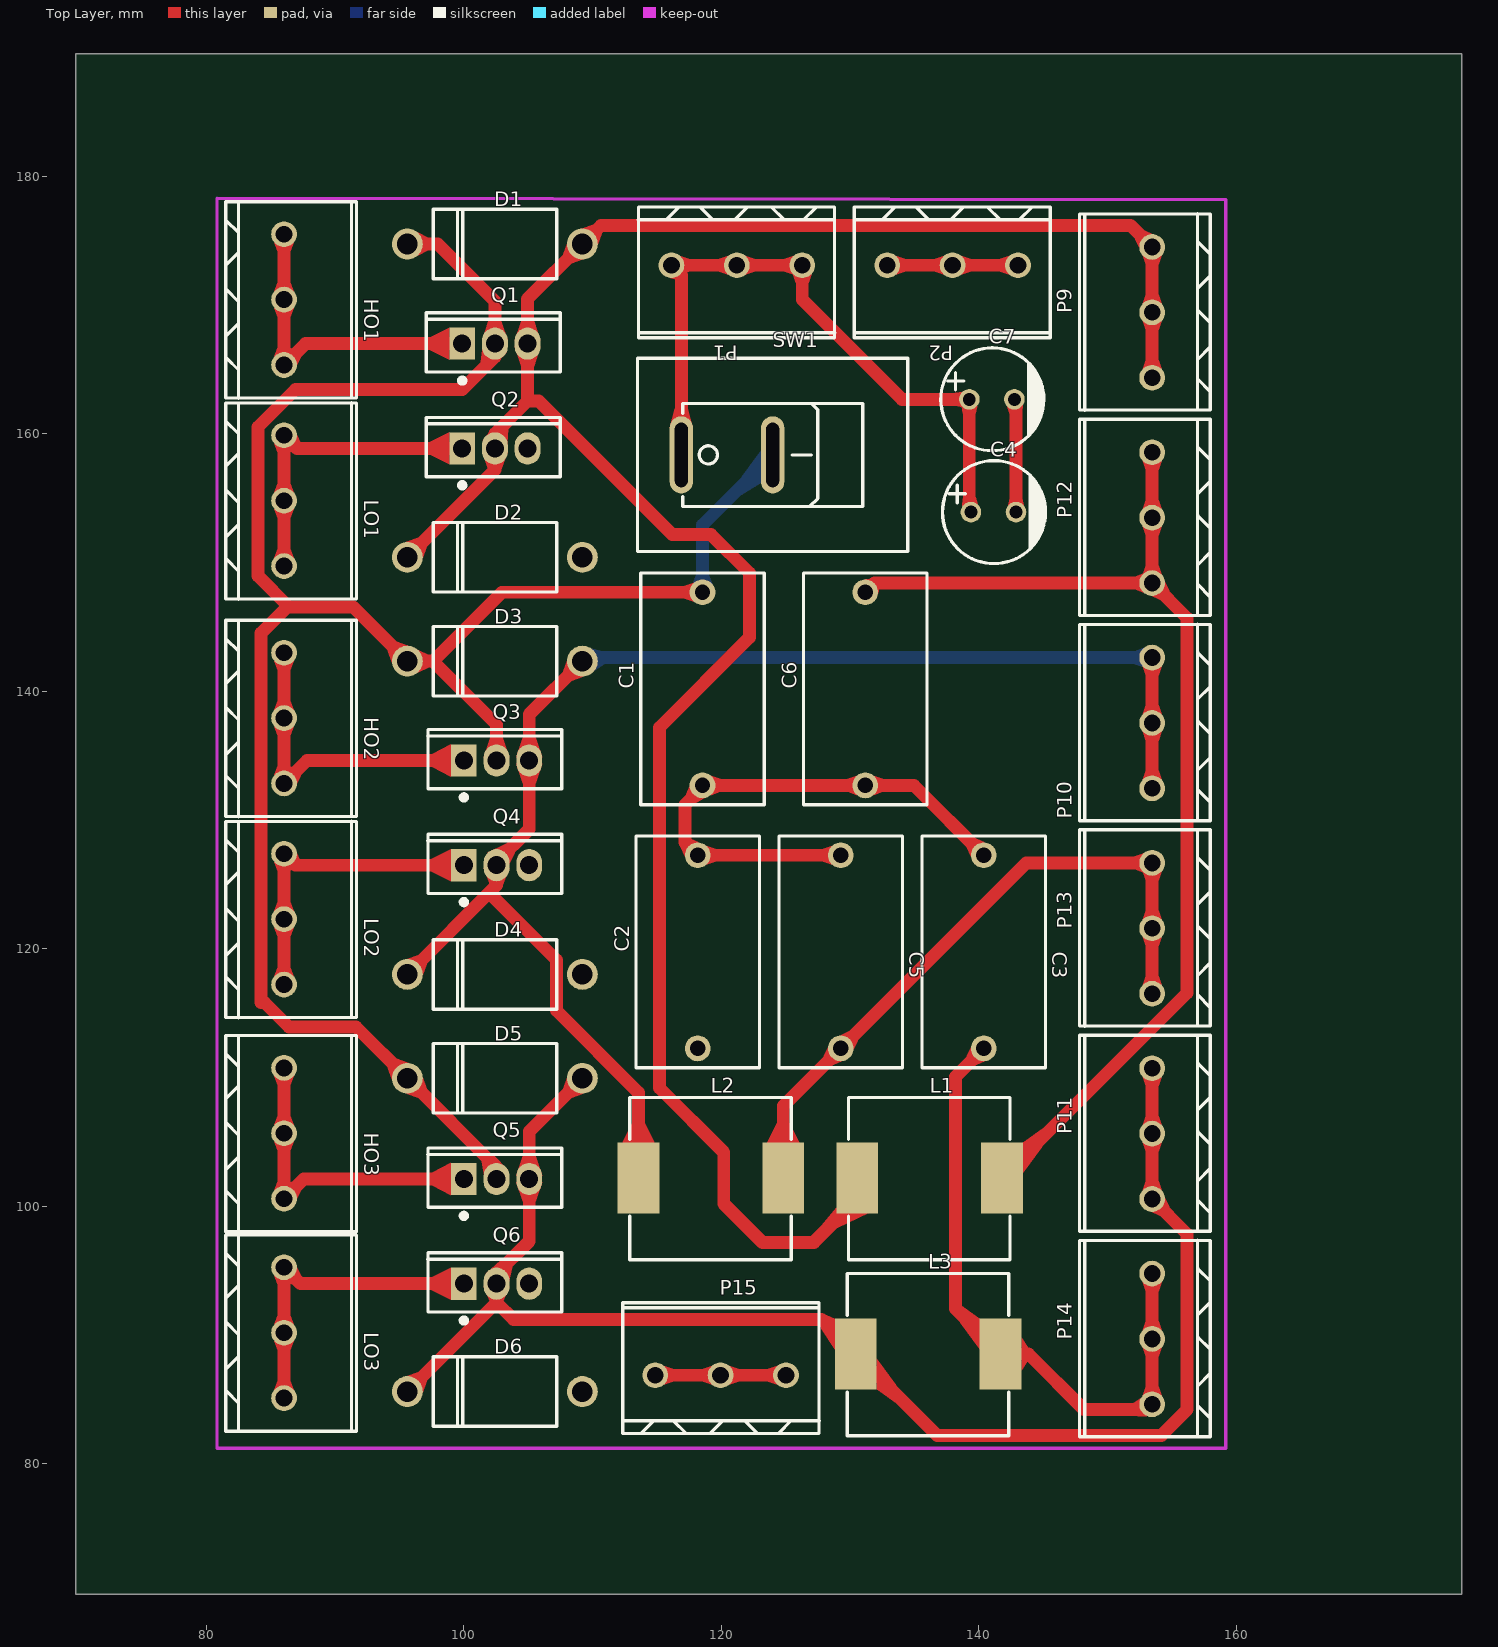
[diagram p0: Top Layer view]
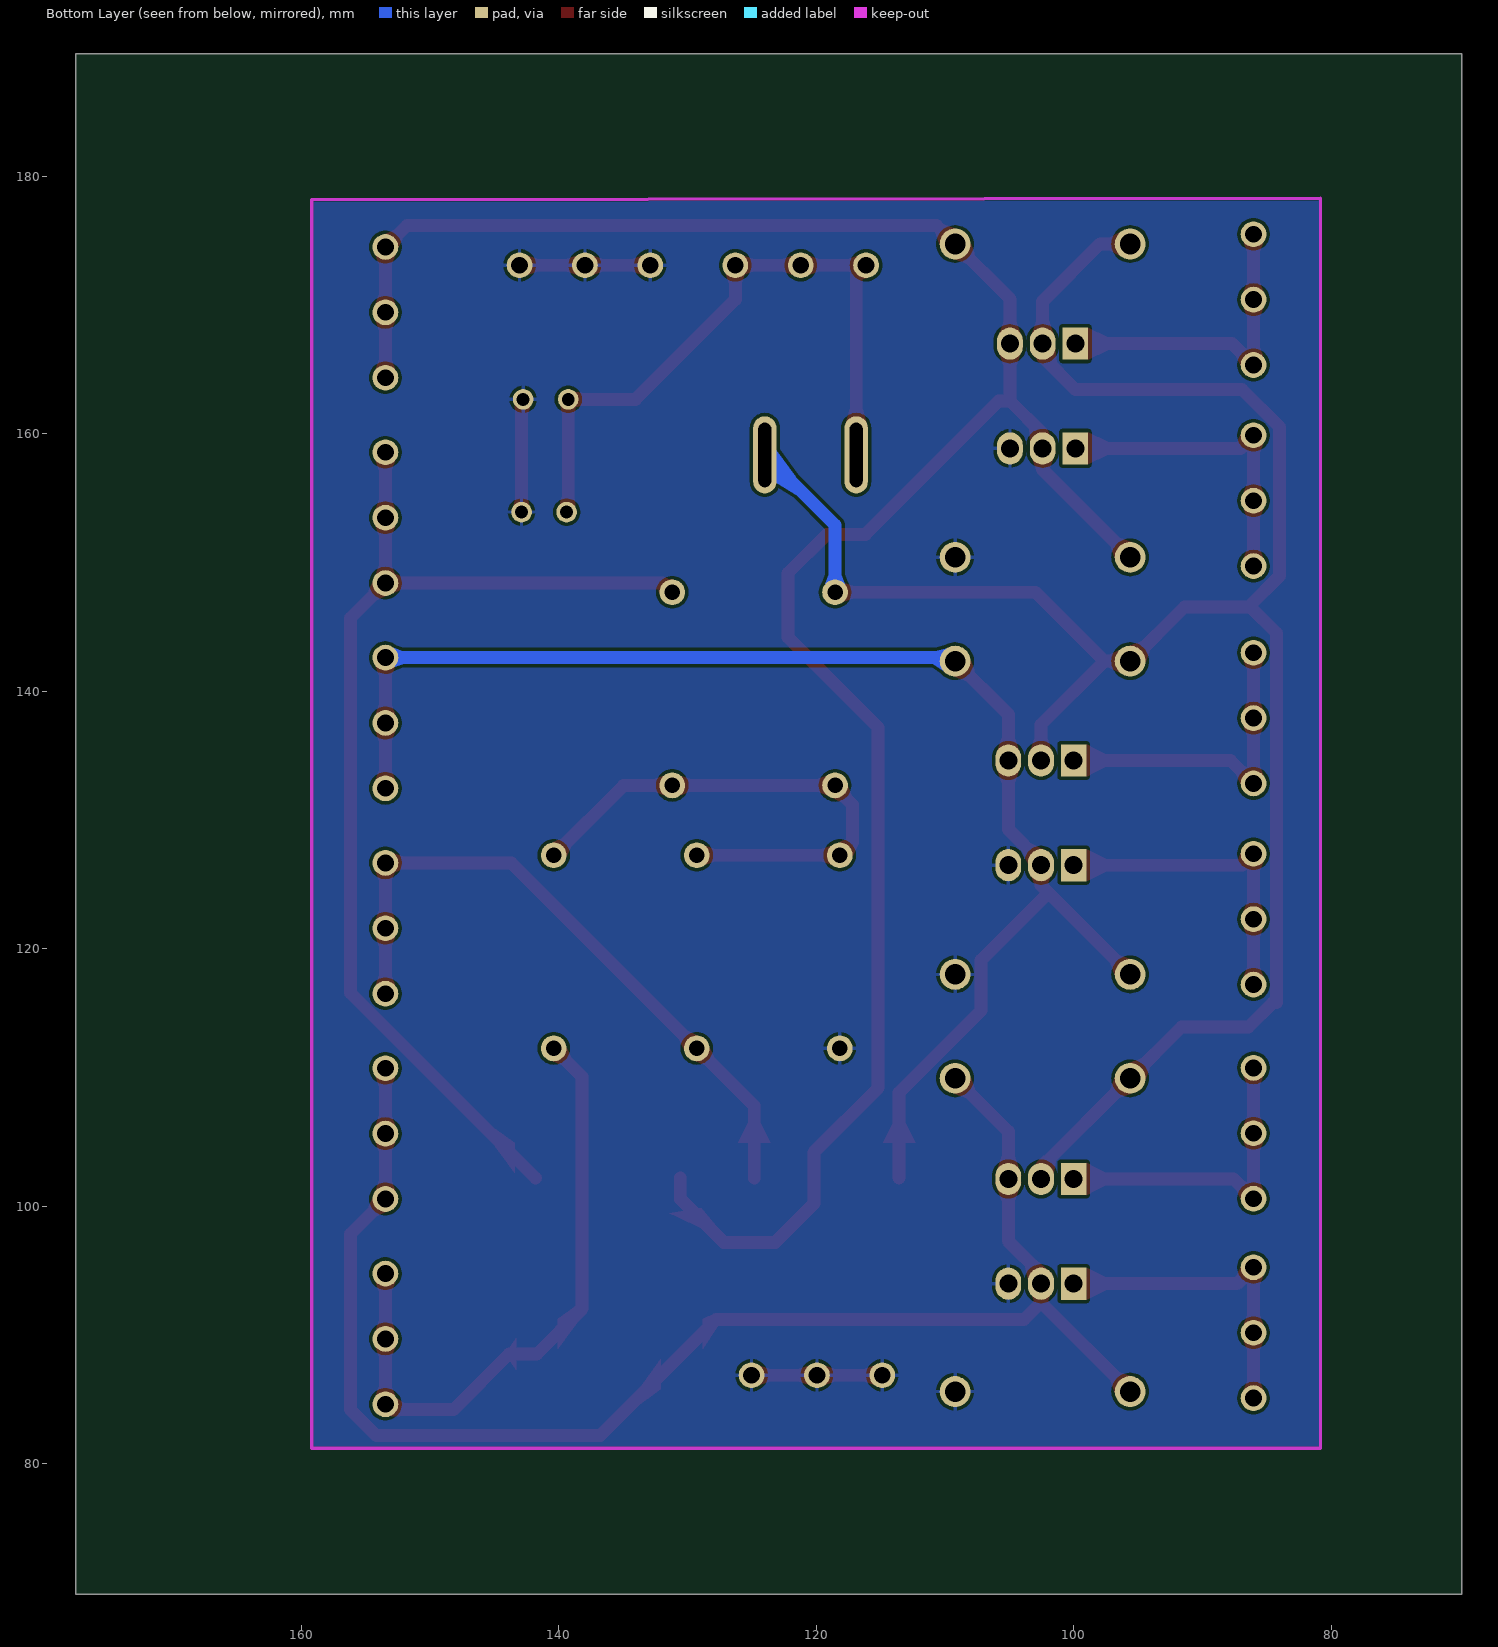
[diagram p1: Bottom Layer view, seen from below]
# Altium PCB MISC75150.pcbdoc
Units mm, origin at the board's own origin, x right, y up, seen from the top; angles counter-clockwise.
Board outline 107.7 x 119.7 mm, 2 copper layers (Top Layer, Bottom Layer), stack 0.07 mm thick; 38 components, 16 nets, 97 pads, 0 vias.

## Layer stack, top to bottom
Top Solder Mask Layer: solder mask 0.01, Dk 3.3
Top Layer: signal copper 0.035
Bottom Layer: signal copper 0.035
Bottom Solder Mask Layer: solder mask 0.01, Dk 3.3

## Board outline
177.55,69.85 69.85,69.85 69.85,189.55 177.55,189.55

## Design rules (kind name [scope] priority, off if disabled: settings)
BoardOutlineClearance Default_1 [All] p2: genericclearance=0.102 ignorepadtopadclearanceinfootprint=FALSE except(0: Arc-SplitContinuation Track-SplitContinuation SMDPad-SplitContinuation THPad-SplitContinuation Via-SplitContinuation Fill-SplitContinuation Region-SplitContinuation Poly-SplitContinuation Text-SplitContinuation Hole-SplitContinuation; 0.152: Arc-OutlineEdge Track-OutlineEdge SMDPad-OutlineEdge THPad-OutlineEdge Via-OutlineEdge Fill-OutlineEdge Region-OutlineEdge Poly-OutlineEdge Text-OutlineEdge Hole-OutlineEdge SMDPad-CutoutEdge THPad-CutoutEdge Via-CutoutEdge Fill-CutoutEdge Region-CutoutEdge Text-CutoutEdge; 0.175: Hole-CutoutEdge; 0.254: Poly-CutoutEdge; 0.3: Arc-CutoutEdge Track-CutoutEdge)
Clearance Default [All] p1: gap=0.102 ignorepadtopadclearanceinfootprint=FALSE except(0.152: SMDPad-Track SMDPad-SMDPad THPad-Track SMDPad-THPad THPad-THPad Track-Via SMDPad-Via THPad-Via Via-Via Fill-Track Region-Track Fill-SMDPad Region-SMDPad Fill-THPad Region-THPad Fill-Via Region-Via Fill-Fill Fill-Region Region-Region Arc-Track Arc-SMDPad Arc-THPad Arc-Via Fill-Arc Region-Arc Arc-Arc Text-Track SMDPad-Text Text-THPad Text-Via Fill-Text Region-Text Arc-Text Text-Text; 0.175: Hole-Track Hole-SMDPad Hole-THPad Hole-Via Fill-Hole Region-Hole Hole-Arc Hole-Text; 0.254: Poly-Track Poly-SMDPad Poly-THPad Poly-Via Poly-Fill Poly-Region Poly-Poly Poly-Arc Poly-Text Poly-Hole)
DiffPairsRouting differentialPair [All] p1: maxlimit=0.152 minlimit=0.127 mostfreqgap=0.152 toplayer_minwidth=0.127 toplayer_prefwidth=2.54 toplayer_maxwidth=2.54 toplayer_mingap=0.127 toplayer_prefgap=0.152 toplayer_maxgap=0.152 bottomlayer_minwidth=0.127 bottomlayer_prefwidth=2.54 bottomlayer_maxwidth=2.54 bottomlayer_mingap=0.127 bottomlayer_prefgap=0.152 bottomlayer_maxgap=0.152 maxuncoupledlength=0.254
HoleToHoleClearance otherClearance [All] p1: gap=0.3 allowstackedmicrovias=TRUE
Length netLength [All] p1: minlimit=0 maxlimit=0
MatchedLengths netLengthTolerance [All] p1: tolerance=25.4
PasteMaskExpansion pasteMaskExpansion [All] p1: expansion=0
PlaneConnect innerPlane [All] p1: planeconnectstyle=Relief reliefexpansion=0.508 reliefentries=4 reliefconductorwidth=0.254 reliefairgap=0.254
PolygonConnect copperRegion [All] p1: connectstyle=Relief reliefconductorwidth=0.254 reliefentries=4 polygonreliefangle="90 Angle" airgapwidth=0.254 via.connectstyle=Relief via.reliefconductorwidth=0.254 via.reliefentries=4 via.polygonreliefangle="90 Angle" via.airgapwidth=0.254
RoutingVias Default_3 [All] p1: holewidth=0.305 width=0.61 viastyle="Through Hole" minholewidth=0.305 minwidth=0.61 maxholewidth=29.997 maxwidth=50.013
SolderMaskExpansion Common [IsVia] p1: expansion=-25.4 istentingtop=TRUE
SolderMaskExpansion Common [All] p2: expansion=0.051 istentingtop=FALSE
Width Default_2 [All] p1: maxlimit=25.4 minlimit=0.254 preferedwidth=0.254

## Components (designator, comment, footprint, x,y, rotation, side; value= is the part's Value field where it differs from the comment)
C1 "1uF" CAP-TH_L18.0-W9.5-P15.00-D1.2 118.551,140.2 r90 top
C2 "1uF" CAP-TH_L18.0-W9.5-P15.00-D1.2 118.18,119.768 r90 top
C3 "1uF" CAP-TH_L18.0-W9.5-P15.00-D1.2 140.405,119.768 r270 top
C4 "100uF, voltage stabilising" CAP-TH_BD8.0-P3.50-D1.0-FD 141.157,153.931 r0 top
C5 "1uF" CAP-TH_L18.0-W9.5-P15.00-D1.2 129.293,119.768 r270 top
C6 "1uF" CAP-TH_L18.0-W9.5-P15.00-D1.2 131.2,140.2 r90 top
C7 "100uF, voltage stabilising" CAP-TH_BD8.0-P3.50-D1.0-FD 141.03,162.694 r0 top
D1 "FR307" DO-201AD_BD5.3-L8.4-P12.50-D1.4-RD 102.422,174.759 r0 top
D2 "FR307" DO-201AD_BD5.3-L8.4-P12.50-D1.4-RD 102.422,150.42 r0 top
D3 "FR307" DO-201AD_BD5.3-L8.4-P12.50-D1.4-RD 102.422,142.352 r0 top
D4 "FR307" DO-201AD_BD5.3-L8.4-P12.50-D1.4-RD 102.422,118.012 r0 top
D5 "FR307" DO-201AD_BD5.3-L8.4-P12.50-D1.4-RD 102.422,109.944 r0 top
D6 "FR307" DO-201AD_BD5.3-L8.4-P12.50-D1.4-RD 102.422,85.605 r0 top
HO1 "First channel high-level control input" CONN-TH_3P-P5.00_WJ500V-5.08-3P 86.039,170.441 r270 top
HO2 "Second channel high-level control input" CONN-TH_3P-P5.00_WJ500V-5.08-3P 86.039,137.929 r270 top
HO3 "Third channel high-level control input" CONN-TH_3P-P5.00_WJ500V-5.08-3P 86.039,105.671 r270 top
L1 "100uH" IND-SMD_L13.5-W12.6_125CDMCC-DS 136.2,102.2 r0 top
L2 "100uH" IND-SMD_L13.5-W12.6_125CDMCC-DS 119.2,102.2 r0 top
L3 "100uH" IND-SMD_L13.5-W12.6_125CDMCC-DS 136.087,88.526 r0 top
LO1 "First channel low-level control input" CONN-TH_3P-P5.00_WJ500V-5.08-3P 86.039,154.82 r270 top
LO2 "Second channel low-level control input" CONN-TH_3P-P5.00_WJ500V-5.08-3P 86.039,122.308 r270 top
LO3 "Third channel low-level control input" CONN-TH_3P-P5.00_WJ500V-5.08-3P 86.039,90.177 r270 top
P1 "DC supply V1 positive" CONN-TH_3P-P5.00_WJ500V-5.08-3P 121.218,173.108 r180 top
P2 "DC supply V1 negative" CONN-TH_3P-P5.00_WJ500V-5.08-3P 137.982,173.108 r180 top
P9 "Provides first channel reference voltage" CONN-TH_3P-P5.00_WJ500V-5.08-3P 153.486,169.45 r90 top
P10 "Provides second channel reference voltage" CONN-TH_3P-P5.00_WJ500V-5.08-3P 153.486,137.548 r90 top
P11 "Provides third channel reference voltage" CONN-TH_3P-P5.00_WJ500V-5.08-3P 153.486,105.646 r90 top
P12 "First channel load" CONN-TH_3P-P5.00_WJ500V-5.08-3P 153.486,153.499 r90 top
P13 "Second channel load" CONN-TH_3P-P5.00_WJ500V-5.08-3P 153.486,121.597 r90 top
P14 "Third channel load" CONN-TH_3P-P5.00_WJ500V-5.08-3P 153.486,89.694 r90 top
P15 "Add ground interface" CONN-TH_3P-P5.00_WJ500V-5.08-3P 119.958,86.875 r0 top
Q1 "IRF540N" TO-220AB-3_L10.4-W4.6-P2.54-L 102.422,167.019 r0 top
Q2 "IRF540N" TO-220AB-3_L10.4-W4.6-P2.54-L 102.422,158.884 r0 top
Q3 "IRF540N" TO-220AB-3_L10.4-W4.6-P2.54-L 102.549,134.634 r0 top
Q4 "IRF540N" TO-220AB-3_L10.4-W4.6-P2.54-L 102.549,126.499 r0 top
Q5 "IRF540N" TO-220AB-3_L10.4-W4.6-P2.54-L 102.549,102.122 r0 top
Q6 "IRF540N" TO-220AB-3_L10.4-W4.6-P2.54-L 102.549,93.987 r0 top
SW1 "MR1-110-C5N-BB" SW-TH_MR1-110-C5N-BB 120.456,158.376 r0 top

## Footprints (in the part's own frame and the unit in brackets; to place one, negate y for a bottom-side part, rotate by r counter-clockwise, add the part's x,y. Pads: shape width x height; smd on the part's side, far side on the other; paste and mask are expansions set on the pad)
CAP-TH_BD8.0-P3.50-D1.0-FD [mm]
  round 1.6 hole 1 paste+0 mask+0.102: 1(-1.75,0) 2(1.75,0)
  Top Layer circle w0.6: c1.75,0 r0.3
  Top Layer circle w0.6: c-1.75,0 r0.3
  silkscreen extent -3.96,-4 4.04,4
CAP-TH_L18.0-W9.5-P15.00-D1.2 [mm]
  round 2 hole 1.2 paste+0 mask+0.102: 1(-7.501,0) 2(7.501,0)
  silkscreen extent -9,-4.8 9,4.8
CONN-TH_3P-P5.00_WJ500V-5.08-3P [mm]
  round 2 hole 1.3 paste+0 mask+0.102: 1(-5.08,0) 2(0,0) 3(5.08,0)
  silkscreen extent -7.61,-4.53 7.66,5.64
DO-201AD_BD5.3-L8.4-P12.50-D1.4-RD [mm]
  round 2.4 hole 1.6 paste+0 mask+0.102: 1(-6.8,0) 2(6.8,0)
  silkscreen extent -4.8,-2.7 4.8,2.7
IND-SMD_L13.5-W12.6_125CDMCC-DS [mm]
  rect 3.25x5.5 smd paste+0 mask+0.102: 1(-5.625,0) 2(5.625,0)
  silkscreen extent -6.3,-6.35 6.25,6.25
SW-TH_MR1-110-C5N-BB [mm]
  oval 1.8x6 hole 1 slot 5 at 90 deg paste+0 mask+0.102: 1(-3.55,0) 2(3.55,0)
  silkscreen extent -6.95,-7.5 14.05,7.5
TO-220AB-3_L10.4-W4.6-P2.54-L [mm]
  rect 2x2.5 hole 1.4 paste+0 mask+0.102: 1(-2.54,0)
  oval 2x2.5 hole 1.4 paste+0 mask+0.102: 2(0,0) 3(2.54,0)
  silkscreen extent -5.33,-3.07 5.08,2.4

## Nets (pads, with @x,y where several pads share a name; then routed paths per layer and width w, separated by ;. In a path a pad name is that pad's centre, name@x,y a point inside that pad or via, vN(x,y) a via of type N, cw(c..) or ccw(c..) an arc to the next point about the centre after c; other vN are vias at no path point)
C1_1: C1.1 C2.2 C3.1 C5.1 C6.1 | length 41.6
  Top Layer w1: C5.1 C2.2 117.2,128.249 117.2,131.2 118.551,132.551 C1.1 C6.1 134.974,132.699 C3.1
C1_2: C1.2 D1.1 D3.1 D5.1 Q1.2 Q3.2 Q5.2 SW1.2 | length 163.6
  Top Layer w1: D5.1 91.64,113.926 86.42,113.926 84.515,115.831 84.261,115.831 84.261,144.533 86.293,146.565 86.42,146.565 ; D5.1 102.549,103.017 Q5.2 ; D1.1 97.977,174.759 102.422,170.314 Q1.2 102.422,165.996 99.882,163.456 86.928,163.456 84.007,160.535 84.007,148.978 86.42,146.565 ; 97.619,142.352 102.968,147.701 C1.2 ; Q3.2 102.549,137.421 97.619,142.351 D3.1 91.409,146.565 86.42,146.565
  Bottom Layer w1: C1.2 118.551,152.92 SW1.2@124.007,158.376
C3_2: C3.2 L3.2 P14.1 P14.2 P14.3 | length 50
  Top Layer w1: C3.2 138.201,110.063 138.201,92.039 L3.2 143.875,88.526 148.201,84.2 153.073,84.2 P14.1 ; P14.1 P14.2 P14.3
C5_2: C5.2 L2.2 P13.1 P13.2 P13.3 | length 52.2
  Top Layer w1: L2.2 124.825,107.8 C5.2 ; C5.2 143.702,126.677 P13.3 P13.2 P13.1
C6_2: C6.2 L1.2 P12.1 P12.2 P12.3 | length 86
  Top Layer w1: C6.2 131.919,148.419 P12.1 P12.2 P12.3 ; L1.2 156.199,116.575 156.199,145.704 P12.1
GND: C2.1 C4.2 C7.2 D2.2 D4.2 D6.2 P2.1 P2.2 P2.3 P15.1 P15.2 P15.3 Q2.3 Q4.3 Q6.3 | length 29.1
  Top Layer w1: P15.1 P15.2 P15.3 ; P2.3 P2.2 P2.1 ; C7.2 142.908,162.567 C4.2
Q1_1: HO1.1 HO1.2 HO1.3 Q1.1 | length 24.7
  Top Layer w1: HO1.1 86.039,172.763 HO1.2 HO1.3 87.698,167.02 Q1.1
Q1_3: D1.2 D2.1 L1.1 P9.1 P9.2 P9.3 Q1.3 Q2.2 | length 177.1
  Top Layer w1: D2.1@95.623,150.421 102.422,157.22 Q2.2 102.422,160.027 104.962,162.567 ; L1.1@130.576,102.199 130.576,100.576 127.2,97.2 123.2,97.2 120.2,100.2 120.2,104.2 115.201,109.199 115.201,137.2 122.199,144.2 122.199,149.199 119.199,152.201 116.199,152.201 105.834,162.567 104.962,162.567 ; P9.1 P9.2 P9.3 151.816,176.2 110.664,176.2 D1.2 104.962,170.499 Q1.3 104.962,162.567
Q2_1: LO1.1 LO1.2 LO1.3 Q2.1 | length 24.4
  Top Layer w1: LO1.3 LO1.2 LO1.1 87.055,158.884 Q2.1
Q3_1: HO2.1 HO2.2 HO2.3 Q3.1 | length 24.9
  Top Layer w1: HO2.1 HO2.3 87.825,134.635 Q3.1
Q3_3: D3.2 D4.1 L2.1 P10.1 P10.2 P10.3 Q3.3 Q4.2 | length 111.5
  Top Layer w1: D4.1 102.549,124.939 Q4.2 102.549,126.753 105.089,129.293 Q3.3 105.089,138.219 D3.2 ; 101.97,124.36 107.2,119.13 107.2,115.201 113.576,108.826 L2.1 ; P10.1 P10.2 P10.3
  Bottom Layer w1: D3.2 109.499,142.628 P10.3
Q4_1: LO2.1 LO2.2 LO2.3 Q4.1 | length 24.5
  Top Layer w1: LO2.3 LO2.2 LO2.1 86.928,126.499 Q4.1
Q5_1: HO3.1 HO3.2 HO3.3 Q5.1 | length 24.8
  Top Layer w1: HO3.1 HO3.2 HO3.3 87.571,102.123 Q5.1
Q5_3: D5.2 D6.1 L3.1 P11.1 P11.2 P11.3 Q5.3 Q6.2 | length 116.4
  Top Layer w1: D6.1 102.549,92.532 ; D5.2 105.089,105.811 Q5.3 105.089,97.289 102.549,94.749 Q6.2 102.549,92.532 ; P11.1 P11.2 P11.3 ; P11.1 156.199,97.853 156.199,84.2 154.2,82.199 136.789,82.199 L3.1 127.787,91.201 103.88,91.201 102.549,92.532
Q6_1: LO3.1 LO3.2 LO3.3 Q6.1 | length 24.7
  Top Layer w1: LO3.3 LO3.2 LO3.1 87.309,93.987 Q6.1
VCC: C4.1 C7.1 P1.1 P1.2 P1.3 SW1.1 | length 52.9
  Top Layer w1: SW1.1 116.906,172.341 P1.3 P1.2 P1.1 126.298,170.441 134.045,162.694 C7.1 139.28,154.058 C4.1

## Polygon pours and split planes (outlines as drawn)
GND on Bottom Layer (solid, remove dead copper, pour order 2): 76.2,183.2 171.2,183.2 170.2,182.2 170.2,76.2 76.2,76.2 76.2,77.2

## Keep-outs
Board Outline Layer:
  lines w0.254: 80.832,81.211 159.2,81.2 159.2,178.2 80.832,178.315 80.832,81.211

## Other copper
Top Layer:
  region net VCC: 116.8,172.358 116.8,173.858 117.5,173.608 117.5,172.608
  region net VCC: 116.076,172.11 117.136,173.171 117.26,172.694 116.553,171.987
  region net VCC: 121.88,172.358 121.88,173.858 122.58,173.608 122.58,172.608
  region net VCC: 120.557,172.358 120.557,173.858 119.857,173.608 119.857,172.608
  region net VCC: 125.637,172.358 125.637,173.858 124.937,173.608 124.937,172.608
  region net VCC: 127.048,172.447 125.548,172.447 125.798,171.747 126.798,171.747
  region net GND: 133.564,172.358 133.564,173.858 134.264,173.608 134.264,172.608
  region net GND: 137.321,172.358 137.321,173.858 136.621,173.608 136.621,172.608
  region net GND: 138.644,172.358 138.644,173.858 139.344,173.608 139.344,172.608
  region net GND: 142.401,172.358 142.401,173.858 141.701,173.608 141.701,172.608
  region net Q1_1: 86.789,166.022 85.289,166.022 85.539,166.722 86.539,166.722
  region net Q1_1: 85.977,166.359 87.037,165.298 87.356,165.97 86.649,166.677
  region net Q1_1: 86.789,171.102 85.289,171.102 85.539,171.802 86.539,171.802
  region net Q1_1: 86.789,169.78 85.289,169.78 85.539,169.08 86.539,169.08
  region net Q1_1: 86.789,174.86 85.289,174.86 85.539,174.16 86.539,174.16
  region net Q2_1: 86.789,150.401 85.289,150.401 85.539,151.101 86.539,151.101
  region net Q2_1: 86.789,155.481 85.289,155.481 85.539,156.181 86.539,156.181
  region net Q2_1: 86.789,154.159 85.289,154.159 85.539,153.459 86.539,153.459
  region net Q2_1: 86.789,159.239 85.289,159.239 85.539,158.539 86.539,158.539
  region net Q2_1: 85.977,158.902 87.037,159.963 87.356,159.291 86.649,158.584
  region net Q3_1: 86.789,133.51 85.289,133.51 85.539,134.21 86.539,134.21
  region net Q3_1: 85.977,133.847 87.037,132.786 87.356,133.458 86.649,134.165
  region net Q3_1: 86.789,137.268 85.289,137.268 85.539,136.568 86.539,136.568
  region net Q3_1: 86.789,138.59 85.289,138.59 85.539,139.29 86.539,139.29
  region net Q3_1: 86.789,142.348 85.289,142.348 85.539,141.648 86.539,141.648
  region net Q4_1: 86.789,117.889 85.289,117.889 85.539,118.589 86.539,118.589
  region net Q4_1: 86.789,122.969 85.289,122.969 85.539,123.669 86.539,123.669
  region net Q4_1: 86.789,121.647 85.289,121.647 85.539,120.947 86.539,120.947
  region net Q4_1: 86.789,126.727 85.289,126.727 85.539,126.027 86.539,126.027
  region net Q4_1: 85.977,126.39 87.037,127.451 87.282,126.853 86.575,126.145
  region net Q5_1: 86.789,101.252 85.289,101.252 85.539,101.952 86.539,101.952
  region net Q5_1: 85.977,101.589 87.037,100.528 87.356,101.2 86.649,101.907
  region net Q5_1: 86.789,106.332 85.289,106.332 85.539,107.032 86.539,107.032
  region net Q5_1: 86.789,105.01 85.289,105.01 85.539,104.31 86.539,104.31
  region net Q5_1: 86.789,110.09 85.289,110.09 85.539,109.39 86.539,109.39
  region net Q6_1: 86.789,85.758 85.289,85.758 85.539,86.458 86.539,86.458
  region net Q6_1: 86.789,90.838 85.289,90.838 85.539,91.538 86.539,91.538
  region net Q6_1: 86.789,89.516 85.289,89.516 85.539,88.816 86.539,88.816
  region net Q6_1: 86.789,94.596 85.289,94.596 85.539,93.896 86.539,93.896
  region net Q6_1: 85.977,94.259 87.037,95.32 87.356,94.648 86.649,93.941
  region net Q1_3: 154.236,173.869 152.736,173.869 152.986,173.169 153.986,173.169
  region net Q1_3: 152.488,174.468 153.549,175.528 152.877,175.847 152.17,175.14
  region net Q1_3: 154.236,168.789 152.736,168.789 152.986,168.089 153.986,168.089
  region net Q1_3: 154.236,170.112 152.736,170.112 152.986,170.812 153.986,170.812
  region net Q1_3: 154.236,165.032 152.736,165.032 152.986,165.732 153.986,165.732
  region net Q3_3: 154.236,141.967 152.736,141.967 152.986,141.267 153.986,141.267
  region net Q3_3: 154.236,138.209 152.736,138.209 152.986,138.909 153.986,138.909
  region net Q3_3: 154.236,136.887 152.736,136.887 152.986,136.187 153.986,136.187
  region net Q3_3: 154.236,133.129 152.736,133.129 152.986,133.829 153.986,133.829
  region net Q5_3: 154.236,110.064 152.736,110.064 152.986,109.364 153.986,109.364
  region net Q5_3: 154.236,106.307 152.736,106.307 152.986,107.007 153.986,107.007
  region net Q5_3: 154.236,104.984 152.736,104.984 152.986,104.284 153.986,104.284
  region net Q5_3: 154.236,101.227 152.736,101.227 152.986,101.927 153.986,101.927
  region net Q5_3: 153.423,99.568 154.484,100.628 154.802,99.957 154.095,99.249
  region net C6_2: 154.236,157.918 152.736,157.918 152.986,157.218 153.986,157.218
  region net C6_2: 154.236,152.838 152.736,152.838 152.986,152.138 153.986,152.138
  region net C6_2: 154.236,154.161 152.736,154.161 152.986,154.861 153.986,154.861
  region net C6_2: 154.236,149.081 152.736,149.081 152.986,149.781 153.986,149.781
  region net C6_2: 152.825,147.669 152.825,149.169 152.125,148.919 152.125,147.919
  region net C6_2: 153.423,147.421 154.484,148.482 154.802,147.81 154.095,147.103
  region net C5_2: 154.236,126.015 152.736,126.015 152.986,125.315 153.986,125.315
  region net C5_2: 152.825,125.927 152.825,127.427 152.125,127.177 152.125,126.177
  region net C5_2: 154.236,122.258 152.736,122.258 152.986,122.958 153.986,122.958
  region net C5_2: 154.236,120.935 152.736,120.935 152.986,120.235 153.986,120.235
  region net C5_2: 154.236,117.178 152.736,117.178 152.986,117.878 153.986,117.878
  region net C3_2: 154.236,94.113 152.736,94.113 152.986,93.413 153.986,93.413
  region net C3_2: 154.236,90.356 152.736,90.356 152.986,91.056 153.986,91.056
  region net C3_2: 154.236,89.033 152.736,89.033 152.986,88.333 153.986,88.333
  region net C3_2: 154.236,85.276 152.736,85.276 152.986,85.976 153.986,85.976
  region net C3_2: 153.084,83.699 152.628,85.127 152.029,84.7 152.349,83.7
  region net GND: 124.377,86.125 124.377,87.625 123.677,87.375 123.677,86.375
  region net GND: 120.619,86.125 120.619,87.625 121.319,87.375 121.319,86.375
  region net GND: 119.297,86.125 119.297,87.625 118.597,87.375 118.597,86.375
  region net GND: 115.539,86.125 115.539,87.625 116.239,87.375 116.239,86.375
  region net C1_1: 119.213,131.949 119.213,133.449 119.913,133.199 119.913,132.199
  region net C1_1: 118.691,131.709 117.552,132.685 117.285,131.992 118.046,131.339
  region net C1_2: 117.89,146.951 117.89,148.451 117.19,148.201 117.19,147.201
  region net C1_1: 117.182,127.206 118.243,128.267 117.571,128.585 116.864,127.878
  region net C1_1: 118.841,126.519 118.841,128.019 119.541,127.769 119.541,126.769
  region net C1_1: 139.407,127.206 140.468,128.267 139.796,128.585 139.089,127.878
  region net C3_2: 139.407,112.33 140.468,111.269 139.796,110.951 139.089,111.658
  region net C1_1: 128.631,126.519 128.631,128.019 127.931,127.769 127.931,126.769
  region net C5_2: 129.23,113.265 130.291,112.205 130.609,112.877 129.902,113.584
  region net C5_2: 128.294,112.33 129.355,111.269 128.683,110.951 127.976,111.658
  region net C1_1: 131.861,131.949 131.861,133.449 132.561,133.199 132.561,132.199
  region net C1_1: 130.539,133.449 130.539,131.949 129.839,132.199 129.839,133.199
  region net C6_2: 131.137,148.699 132.198,147.638 132.272,148.066 131.565,148.773
  region net GND: 142.246,162.099 143.438,162.238 143.408,161.671 142.408,161.554
  region net VCC: 138.751,162.094 138.751,163.294 138.191,163.194 138.191,162.194
  region net VCC: 139.88,162.165 138.68,162.165 138.78,161.605 139.78,161.605
  region net Q1_3: 109.298,173.561 108.025,174.834 107.714,173.957 108.421,173.25
  region net Q1_3: 110.42,174.684 109.147,175.957 110.024,176.268 110.731,175.561
  region net C1_2: 96.416,173.859 96.416,175.659 97.256,175.259 97.256,174.259
  region net Q1_3: 96.82,150.345 95.547,151.618 96.424,151.929 97.131,151.222
  region net Q3_3: 109.298,141.154 108.025,142.427 107.714,141.55 108.421,140.843
  region net C1_2: 96.416,143.252 96.416,141.452 97.256,141.852 97.256,142.852
  region net C1_2: 95.697,143.549 94.425,142.276 94.114,143.153 94.821,143.86
  region net Q3_3: 96.82,117.937 95.547,119.21 96.424,119.521 97.131,118.814
  region net Q5_3: 109.298,108.746 108.025,110.019 107.714,109.142 108.421,108.435
  region net C1_2: 96.82,110.019 95.547,108.746 96.424,108.435 97.131,109.142
  region net C1_2: 95.698,111.142 94.425,109.869 94.114,110.746 94.821,111.453
  region net Q5_3: 96.82,85.53 95.547,86.803 96.424,87.114 97.131,86.407
  region net GND: 143.508,154.46 142.308,154.46 142.408,155.02 143.408,155.02
  region net VCC: 139.942,154.527 138.75,154.387 138.78,154.954 139.78,155.071
  region net Q1_1: 98.882,165.77 98.882,168.269 97.382,167.519 97.382,166.519
  region net Q2_1: 98.882,157.634 98.882,160.134 97.382,159.384 97.382,158.384
  region net Q3_1: 99.009,133.385 99.009,135.884 97.509,135.134 97.509,134.134
  region net Q4_1: 99.009,125.249 99.009,127.749 97.509,126.999 97.509,125.999
  region net Q5_1: 99.009,100.873 99.009,103.372 97.509,102.622 97.509,101.622
  region net Q6_1: 99.009,92.737 99.009,95.237 97.509,94.487 97.509,93.487
  region net Q1_3: 131.414,99.45 128.95,99.873 127.835,98.542 129.042,98.335
  region net C6_2: 143.45,104.95 143.45,102.575 144.95,104.618 144.95,106.032
  region net Q3_3: 112.325,104.95 114.825,104.95 114.075,106.45 113.075,106.45
  region net C5_2: 123.575,104.95 126.075,104.95 125.325,106.45 124.325,106.45
  region net Q5_3: 132.087,88.151 132.087,85.776 133.587,84.694 133.587,86.108
  region net Q5_3: 128.837,88.901 128.837,91.276 128.141,91.554 127.788,90.493
  region net C3_2: 143.337,89.776 143.337,87.276 143.874,88.026 143.874,89.026
  region net C3_2: 140.087,88.901 140.087,91.276 138.587,92.358 138.587,90.944
  region net C1_2: 103.422,167.269 101.422,167.269 101.922,168.769 102.922,168.769
  region net C1_2: 103.339,166.369 101.506,167.17 101.329,165.61 102.313,165.18
  region net Q1_3: 105.962,167.269 103.962,167.269 104.462,168.769 105.462,168.769
  region net Q1_3: 105.962,166.769 103.962,166.769 104.462,165.269 105.462,165.269
  region net Q1_3: 103.362,158.79 101.483,159.478 102.42,160.732 103.456,160.353
  region net Q1_3: 103.422,158.634 101.422,158.634 101.922,157.22 102.922,157.22
  region net C1_2: 103.549,134.884 101.549,134.884 102.049,136.384 103.049,136.384
  region net Q3_3: 106.089,134.384 104.089,134.384 104.589,132.884 105.589,132.884
  region net Q3_3: 106.089,134.884 104.089,134.884 104.589,136.384 105.589,136.384
  region net Q3_3: 103.258,126.043 101.841,127.455 103.254,128.165 103.962,127.459
  region net Q3_3: 103.549,126.249 101.549,126.249 102.049,124.94 103.049,124.94
  region net C1_2: 103.438,102.831 101.661,101.914 101.395,103.464 102.328,103.946
  region net Q5_3: 106.089,101.872 104.089,101.872 104.589,100.372 105.589,100.372
  region net Q5_3: 106.089,102.372 104.089,102.372 104.589,103.872 105.589,103.872
  region net Q5_3: 103.406,93.721 101.693,94.753 102.881,95.788 103.764,95.257
  region net Q5_3: 103.549,93.737 101.549,93.737 102.049,92.532 103.049,92.532
  region net VCC: 117.806,160.476 116.006,160.476 116.406,161.976 117.406,161.976
Bottom Layer:
  region net Q3_3: 152.825,141.878 152.825,143.378 152.125,143.128 152.125,142.128
  region net C1_2: 119.301,148.362 117.801,148.362 118.051,149.062 119.051,149.062
  region net Q3_3: 110.157,141.599 109.853,143.373 110.747,143.128 110.919,142.128
  region net C1_2: 123.108,156.226 123.107,158.726 121.607,156.683 121.607,155.269